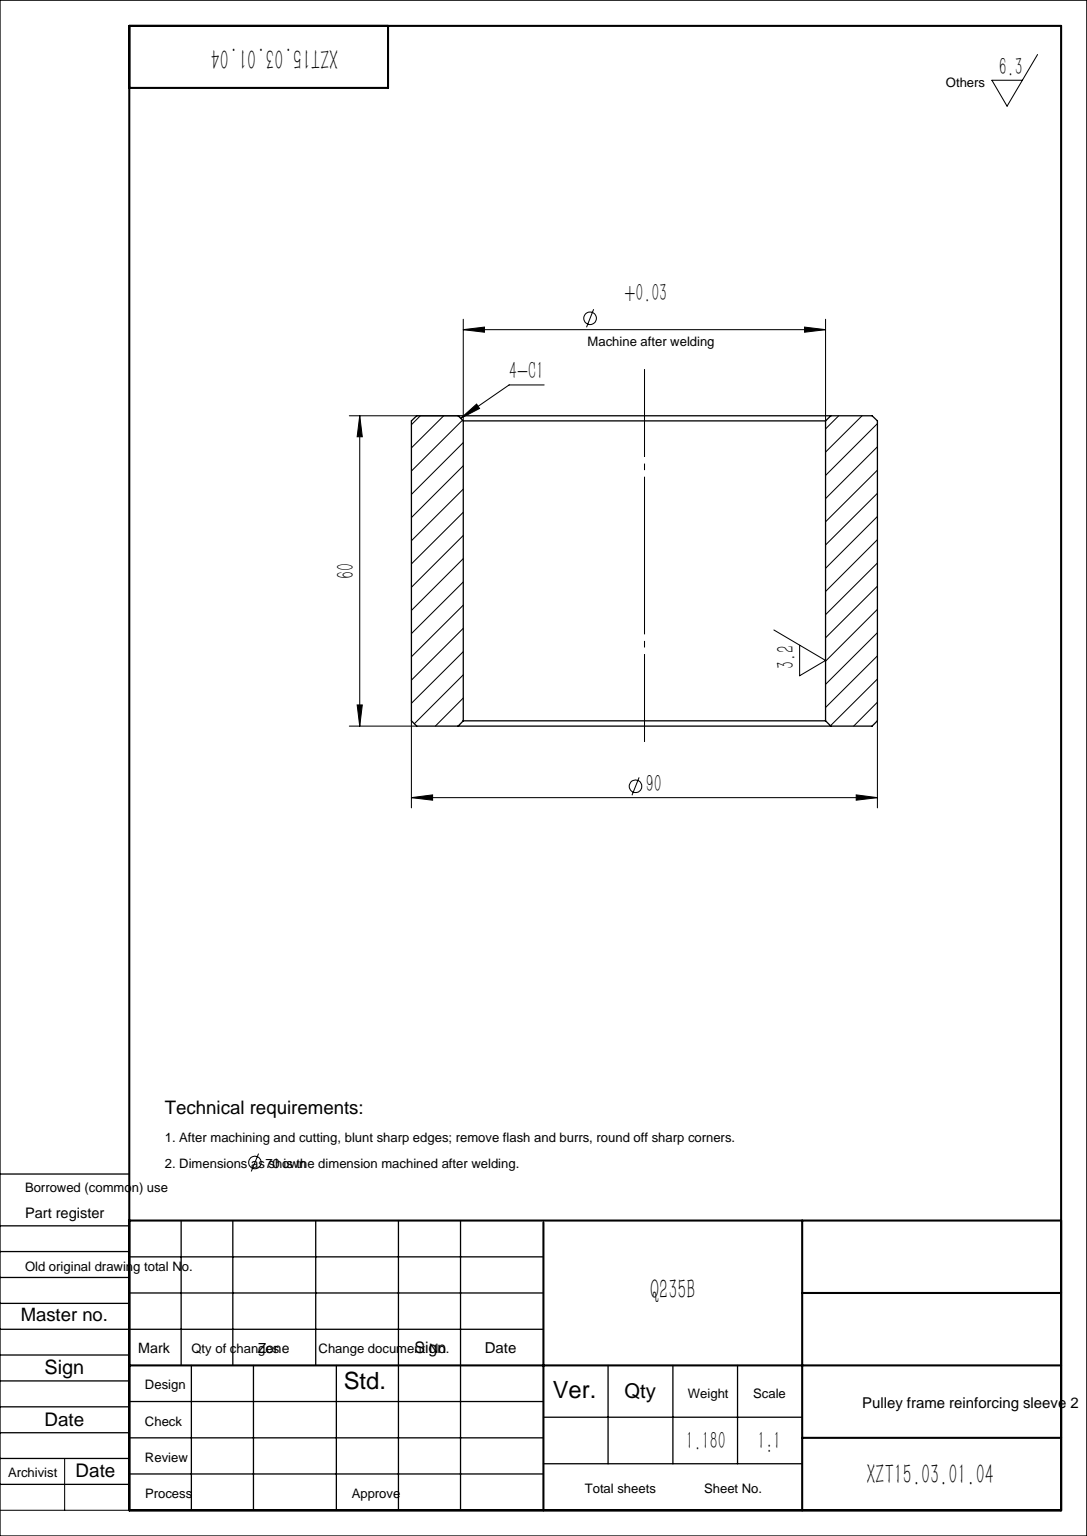
SolidWorks part; units mm, degrees
material "Q235B"
ref_plane "Front Plane" through (0, 0, 0) normal (0, 0, 1) x (1, 0, 0)
ref_plane "Top Plane" through (0, 0, 0) normal (0, 1, 0) x (1, 0, 0)
ref_plane "Right Plane" through (0, 0, 0) normal (1, 0, 0) x (0, 0, -1)
sketch "Sketch1" plane through (0, 0, 0) normal (0, 1, 0) x (1, 0, 0)
  circle A0 centre (0, 0) radius 35
  circle A1 centre (0, 0) radius 45
  dimension "D1" = 70
  dimension "D2" = 90
extrude "Boss-Extrude1" add sketch "Sketch1" along normal blind 60
chamfer "Chamfer2" distance 1 angle 45 4 edges at (0, 0, 35) (0, 60, 35) (0, 0, 45) (0, 60, 45)
